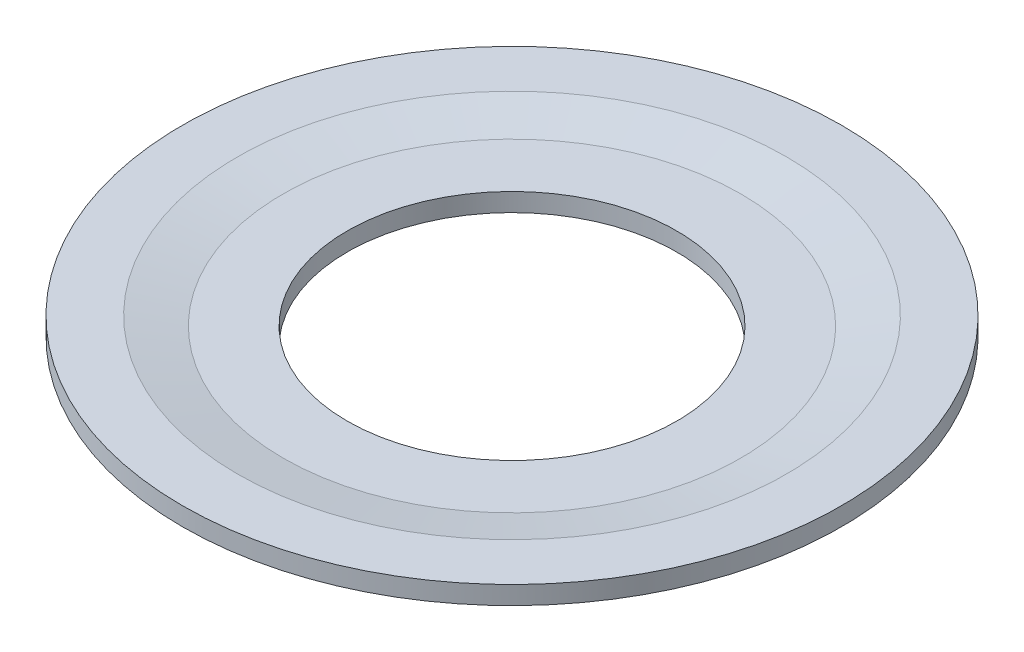
from build123d import *

# Parameters (mm, degrees)
SCALE_1_SCALE = 1.875


with BuildPart() as part:
    # Sketch1 → Revolve1 (revolve)
    with BuildSketch(Plane.XY, mode=Mode.PRIVATE) as revolve1_sk:
        Polygon((0, 0), (0, 2), (7, 2), (12, 2.997347898), (18, 2.997347898), (18, 1), (12, 1), (6, 0), align=None)
    revolve(revolve1_sk.sketch.rotate(Axis((-18, 6.77671814, 0), (0, -1, 0)), 90), axis=Axis((-18, 6.77671814, 0), (0, -1, 0)))


with BuildPart() as part_1:
    # Scale 1: scaled about (-18, 1.56874625, 0)
    add(part.part.scale(SCALE_1_SCALE).moved(Location((15.75, -1.372652969, 0))))


solid = part_1.part
